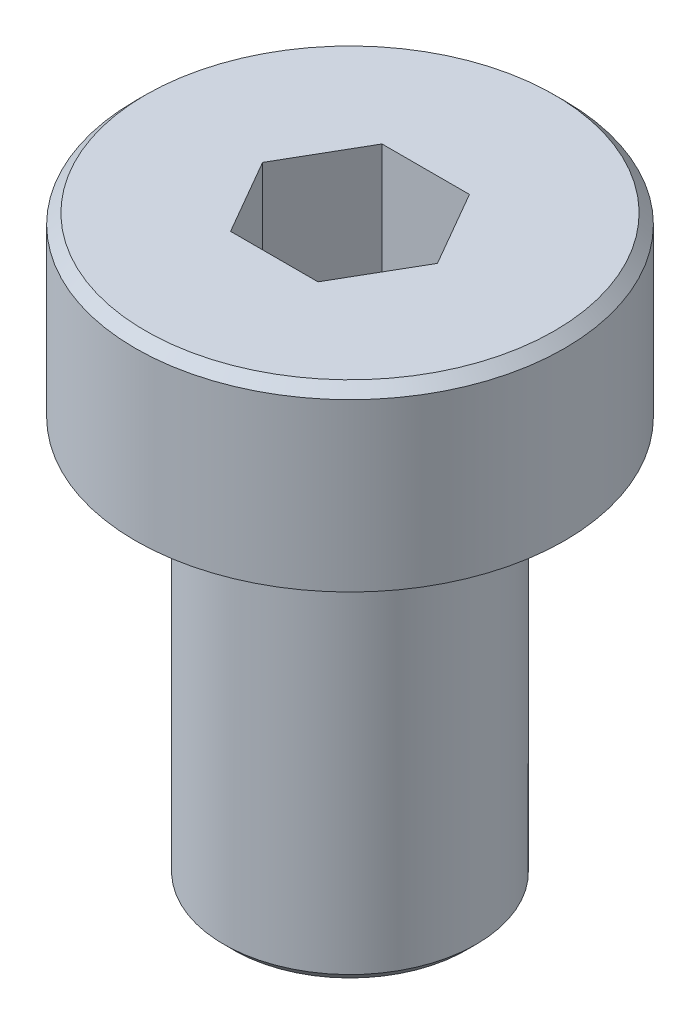
SolidWorks part; units mm, degrees
ref_plane "Front Plane" through (0, 0, 0) normal (0, 0, 1) x (1, 0, 0)
ref_plane "Top Plane" through (0, 0, 0) normal (0, 1, 0) x (1, 0, 0)
ref_plane "Right Plane" through (0, 0, 0) normal (1, 0, 0) x (0, 0, -1)
sketch "Sketch1" plane through (0, 0, 0) normal (0, 0, 1) x (1, 0, 0)
  line L0 (0, 0) -> (0, 8) construction
  line L1 (2.5, 0) -> (4.25, 0)
  line L2 (2.5, 0) -> (2.5, 8)
  line L3 (2.5, 8) -> (0, 8)
  line L6 (1.5, -3.5) -> (1.5, -0.8)
  line L7 (1.5, -0.8) -> (0, 0.066)
  line L11 (2.5, 0) -> (4.25, 0)
  line L12 (4.25, 0) -> (4.25, -3.5)
  line L13 (4.25, -3.5) -> (0, -3.5)
  point P7 (2.5, 0)
  dimension "D1" = 60
  dimension "M" = 5
  dimension "L" = 8
  dimension "t" = 2.7
  dimension "B" = 3
  dimension "E" = 3.5
  dimension "A" = 8.5
  dimension "(l)" = 8
sketch "Sketch2" plane through (0, 0, 0) normal (0, 0, 1) x (1, 0, 0)
  line L0 (1.5, -3.5) -> (1.5, -0.8) construction
  line L1 (1.5, -0.8) -> (0, 0.066) construction
  line L3 (2.5, 0) -> (2.5, 8) construction
  line L4 (2.5, 0) -> (4.25, 0) construction
  line L7 (1.5, -3.5) -> (1.5, -0.8)
  line L8 (1.5, -0.8) -> (0, 0.066)
  line L9 (4.25, 0) -> (4.25, -3.5) construction
  line L10 (2.5, 0) -> (2.5, 8)
  line L14 (0, 0.066) -> (0, 8)
  line L16 (2.5, 8) -> (0, 8) construction
  line L19 (2.5, 8) -> (0, 8)
  line L20 (4.25, -3.5) -> (0, -3.5) construction
  line L21 (2.5, 0) -> (4.25, 0)
  line L22 (4.25, 0) -> (4.25, -3.5)
  line L23 (4.25, -3.5) -> (1.5, -3.5)
revolve "Revolve1" add sketch "Sketch2" angle 360 mid plane about L14
cosmetic thread "Cosmetic Thread1" parameters "D1"=8, "D2"=4.4
chamfer "Chamfer1" distance 0.2 angle 45 2 edges at (2.5, 8, 0) (4.25, -3.5, 0)
sketch "Sketch3" plane through (0, -3.5, 0) normal (0, -1, 0) x (1, 0, 0)
  line L1 (-0.866, 1.5) -> (-1.7321, 0)
  line L2 (-1.7321, 0) -> (-0.866, -1.5)
  line L3 (-0.866, -1.5) -> (0.866, -1.5)
  line L4 (0.866, -1.5) -> (1.7321, 0)
  line L5 (1.7321, 0) -> (0.866, 1.5)
  line L6 (0.866, 1.5) -> (-0.866, 1.5)
  circle A0 centre (0, 0) radius 1.5 construction
extrude "Cut-Extrude1" cut sketch "Sketch3" against normal up to vertex (2.7 mm away) up to point (1.5, -0.8, 0)
move or copy body "Body-Move/Copy1" bodies to move or copy 102 copy no rotation origin (0, 3.25, 0) rotation axis (1, 0, 0) rotation angle 180
